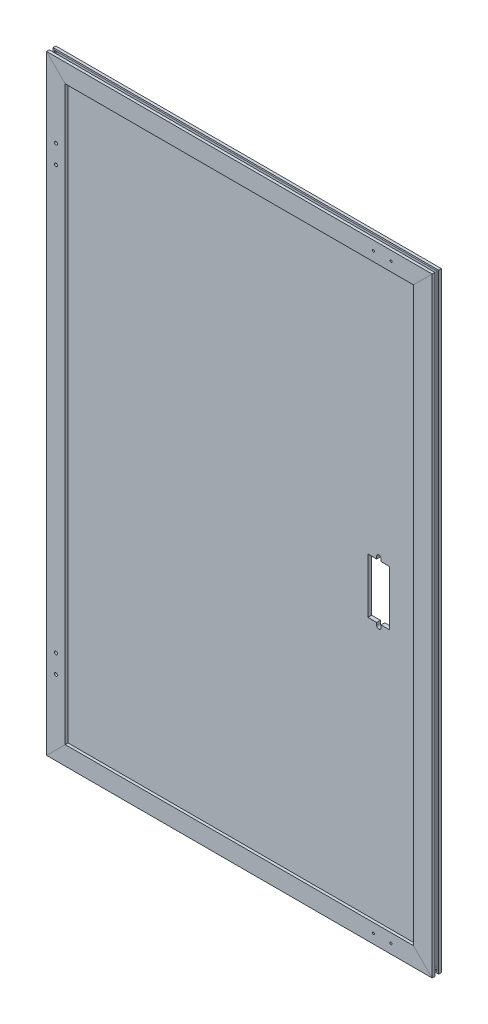
SolidWorks part; units mm, degrees
ref_plane "Front" through (0, 0, 0) normal (0, 0, 1) x (1, 0, 0)
ref_plane "Top" through (0, 0, 0) normal (0, 1, 0) x (1, 0, 0)
ref_plane "Right" through (0, 0, 0) normal (1, 0, 0) x (0, 0, -1)
sketch3d "3DSketch1"
  line L1 (294.25, 474, 0) -> (-294.25, 474, 0)
  line L2 (294.25, 474, 0) -> (294.25, -474, 0)
  line L3 (294.25, -474, 0) -> (-294.25, -474, 0)
  line L4 (-294.25, 474, 0) -> (-294.25, -474, 0)
  line L5 (294.25, 474, 0) -> (-294.25, -474, 0) construction
  line L6 (294.25, -474, 0) -> (-294.25, 474, 0) construction
  point P0 (0, 0, 0)
  dimension "D1" = 588.5
  dimension "D2" = 948
other "Aluminum profile 1530(1)"
ref_plane "Plane1" through (-294.25, 474, 0) normal (0, -1, 0) x (1, 0, 0)
sketch "Sketch1" plane through (-294.25, 474, 0) normal (0, -1, 0) x (1, 0, 0)
  line L4 (-15, -3) -> (-15, -7.5)
  line L5 (-15, -3) -> (-12.5, -3)
  line L6 (-15, -7.5) -> (15, -7.5)
  line L7 (-12.5, -3) -> (-12.5, -5)
  line L8 (15, -3) -> (15, -7.5)
  line L9 (-12.5, -5) -> (-7, -5)
  line L10 (15, -3) -> (12.5, -3)
  line L11 (-7, -5) -> (-7, -3)
  line L12 (12.5, -3) -> (12.5, -5)
  line L13 (-7, -3) -> (-4.5, -3)
  line L14 (12.5, -5) -> (7, -5)
  line L15 (-4.5, -3) -> (-4.5, 3)
  line L16 (7, -5) -> (7, -3)
  line L17 (-4.5, 3) -> (-7, 3)
  line L18 (7, -3) -> (4.5, -3)
  line L19 (-7, 3) -> (-7, 5)
  line L20 (4.5, -3) -> (4.5, 3)
  line L21 (-7, 5) -> (-12.5, 5)
  line L22 (4.5, 3) -> (7, 3)
  line L23 (-12.5, 5) -> (-12.5, 3)
  line L24 (7, 3) -> (7, 5)
  line L25 (-12.5, 3) -> (-15, 3)
  line L26 (7, 5) -> (12.5, 5)
  line L27 (-15, 7.5) -> (-15, 3)
  line L28 (12.5, 5) -> (12.5, 3)
  line L29 (15, 7.5) -> (-15, 7.5)
  line L30 (12.5, 3) -> (15, 3)
  line L31 (15, 7.5) -> (15, 3)
  circle A0 centre (0, 0) radius 2.5
  point P0 (0, 0)
other "Trim/Extend1"
other "Trim/Extend2"
other "Trim/Extend3"
other "Trim/Extend4"
sketch "Sketch2" plane through (0, 0, 0) normal (0, 0, 1) x (1, 0, 0)
  line L0 (-309.25, 489) -> (-279.25, 459) construction
  line L1 (289.25, -469) -> (-289.25, -469)
  line L2 (289.25, -469) -> (289.25, 469)
  line L3 (289.25, 469) -> (-289.25, 469)
  line L4 (-289.25, -469) -> (-289.25, 469)
  line L5 (289.25, -469) -> (-289.25, 469) construction
  line L6 (289.25, 469) -> (-289.25, -469) construction
  line L7 (-279.25, 459) -> (279.25, 459) construction
  point P0 (0, 0)
  dimension "D1" = 10
extrude "Boss-Extrude1" add sketch "Sketch2" along normal mid plane 6 separate body
sketch "Sketch3" plane through (0, 0, 3) normal (0, 0, 1) x (1, 0, 0)
  line L0 (219.25, -48) -> (219.25, 48) construction
  line L1 (201.75, -44) -> (236.75, -44)
  line L2 (201.75, -44) -> (201.75, 44)
  line L3 (201.75, 44) -> (236.75, 44)
  line L4 (236.75, -44) -> (236.75, 44)
  line L5 (201.75, -44) -> (236.75, 44) construction
  line L6 (201.75, 44) -> (236.75, -44) construction
  line L7 (215.75, -48) -> (215.75, 48)
  line L8 (222.75, -48) -> (222.75, 48)
  line L9 (219.25, 0) -> (-279.25, 0) construction
  line L10 (-279.25, -459) -> (-279.25, 459) construction
  line L11 (279.25, -459) -> (279.25, 459) construction
  arc A0 (215.75, -48) -> (222.75, -48) centre (219.25, -48) ccw
  arc A1 (222.75, 48) -> (215.75, 48) centre (219.25, 48) ccw
  point P0 (219.25, 0)
  point P7 (219.25, 0)
  dimension "D4" = 3.5
  dimension "D1" = 60
  dimension "D2" = 35
  dimension "D3" = 88
  dimension "D5" = 96
extrude "Cut-Extrude1" cut sketch "Sketch3" against normal through all contours L4 L3 L2 L1 | A1 L7 A0 L8
hole_wizard "M6 Tapped Hole1" positions "Sketch4" profile "Sketch5" tap size "M6" standard "GB" end condition through all
sketch "Sketch4" plane through (0, 0, 7.5) normal (0, 0, 1) x (1, 0, 0)
  line L0 (-294.25, 369) -> (-294.25, 339)
  line L1 (-294.25, 339) -> (-294.25, -339)
  line L2 (-294.25, -339) -> (-294.25, -369)
  line L4 (-294.25, 0) -> (0, 0)
  line L5 (-309.25, 489) -> (309.25, 489) construction
  line L6 (-309.25, -489) -> (-309.25, 489) construction
  point P0 (-294.25, 369)
  point P2 (-294.25, 339)
  point P4 (-294.25, -339)
  point P6 (-294.25, -369)
  dimension "D1" = 120
  dimension "D2" = 15
  dimension "D3" = 30
sketch "Sketch5" plane through (-294.25, 369, 7.5) normal (1, 0, 0) x (0, -1, 0)
  line L0 (0, 0) -> (0, 15)
  line L1 (0, 15) -> (2.5, 15)
  line L2 (2.5, 15) -> (2.5, 0)
  line L5 (2.5, 0) -> (0, 0)
  line L11 (0, -6.35) -> (0, 107.95) construction
  dimension "通孔螺纹孔钻头直径" = 5
  dimension "通孔螺纹孔钻头深度" = 15
cosmetic thread "Hole-Thread1" parameters "D2"=6
cosmetic thread "Hole-Thread2" parameters "D2"=6
cosmetic thread "Hole-Thread3" parameters "D2"=6
cosmetic thread "Hole-Thread4" parameters "D2"=6
hole_wizard "M4 Tapped Hole1" positions "Sketch6" profile "Sketch7" tap size "M4" standard "GB"
sketch "Sketch6" plane through (0, 0, 7.5) normal (0, 0, 1) x (1, 0, 0)
  line L1 (215.25, -474) -> (243.25, -474)
  line L2 (215.25, -474) -> (215.25, 474)
  line L3 (215.25, 474) -> (243.25, 474)
  line L4 (243.25, -474) -> (243.25, 474)
  line L5 (-309.25, -489) -> (309.25, -489) construction
  line L6 (243.25, 0) -> (309.25, 0)
  line L7 (309.25, -489) -> (309.25, 489) construction
  point P0 (215.25, 474)
  point P2 (243.25, 474)
  point P4 (215.25, -474)
  point P6 (243.25, -474)
  point P66 (229.25, 474)
  dimension "D1" = 28
  dimension "D2" = 15
  dimension "D3" = 80
sketch "Sketch7" plane through (215.25, 474, 7.5) normal (1, 0, 0) x (0, -1, 0)
  line L0 (0, 0) -> (0, 12.4914)
  line L1 (0, 12.4914) -> (1.65, 11.5)
  line L2 (1.65, 11.5) -> (1.65, 0)
  line L5 (1.65, 0) -> (0, 0)
  line L10 (0, 12.4914) -> (-1.65, 11.5) construction
  line L11 (0, -6.35) -> (0, 107.95) construction
  dimension "螺纹孔钻头直径" = 3.3
  dimension "螺纹孔钻头深度" = 11.5
  dimension "导头角度" = 118
cosmetic thread "Hole-Thread5" parameters "D1"=8, "D2"=4
cosmetic thread "Hole-Thread6" parameters "D1"=8, "D2"=4
cosmetic thread "Hole-Thread7" parameters "D1"=8, "D2"=4
cosmetic thread "Hole-Thread8" parameters "D1"=8, "D2"=4
